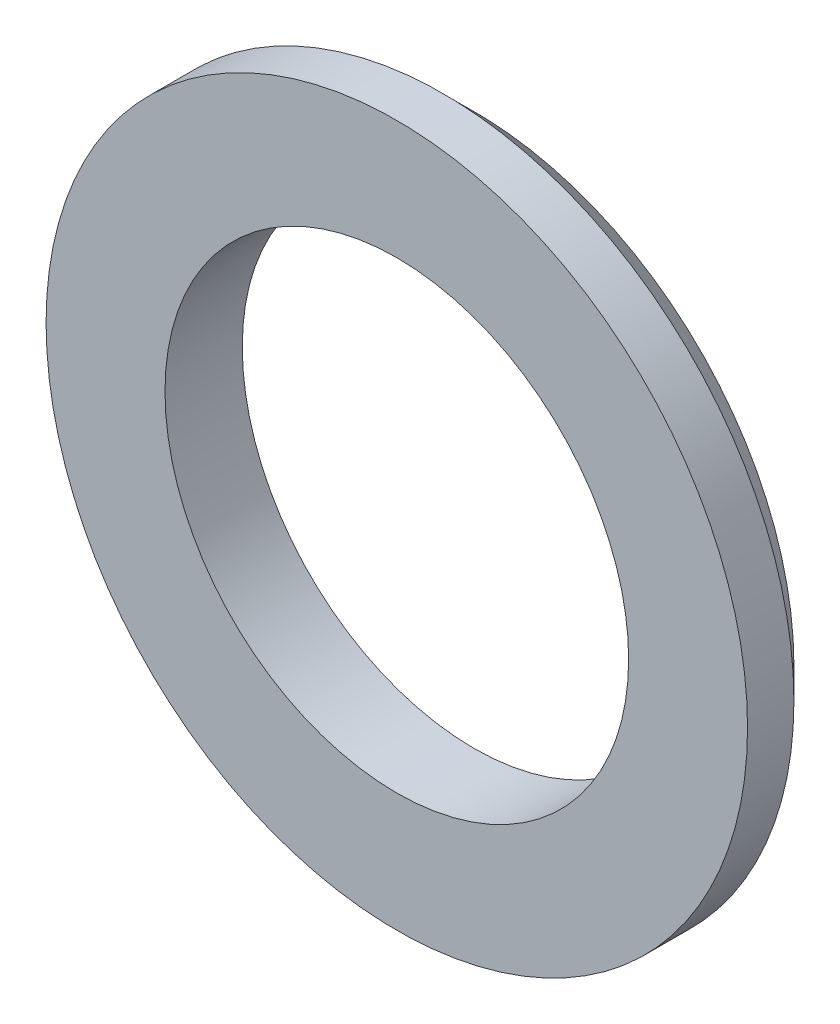
SolidWorks part; units mm, degrees
ref_plane "Front Plane" through (0, 0, 0) normal (0, 0, 1) x (1, 0, 0)
ref_plane "Top Plane" through (0, 0, 0) normal (0, 1, 0) x (1, 0, 0)
ref_plane "Right Plane" through (0, 0, 0) normal (1, 0, 0) x (0, 0, -1)
other "Configuration Table"
sketch "Sketch2" plane through (0, 0, 0) normal (0, 0, 1) x (1, 0, 0)
  circle A0 centre (70, -13) radius 22.6937
  circle A1 centre (70, -13) radius 15
extrude "Boss-Extrude1" add sketch "Sketch2" along normal blind 5
chamfer "Chamfer1" distance 2 angle 45 1 edges at (92.6937, -13, 0)
